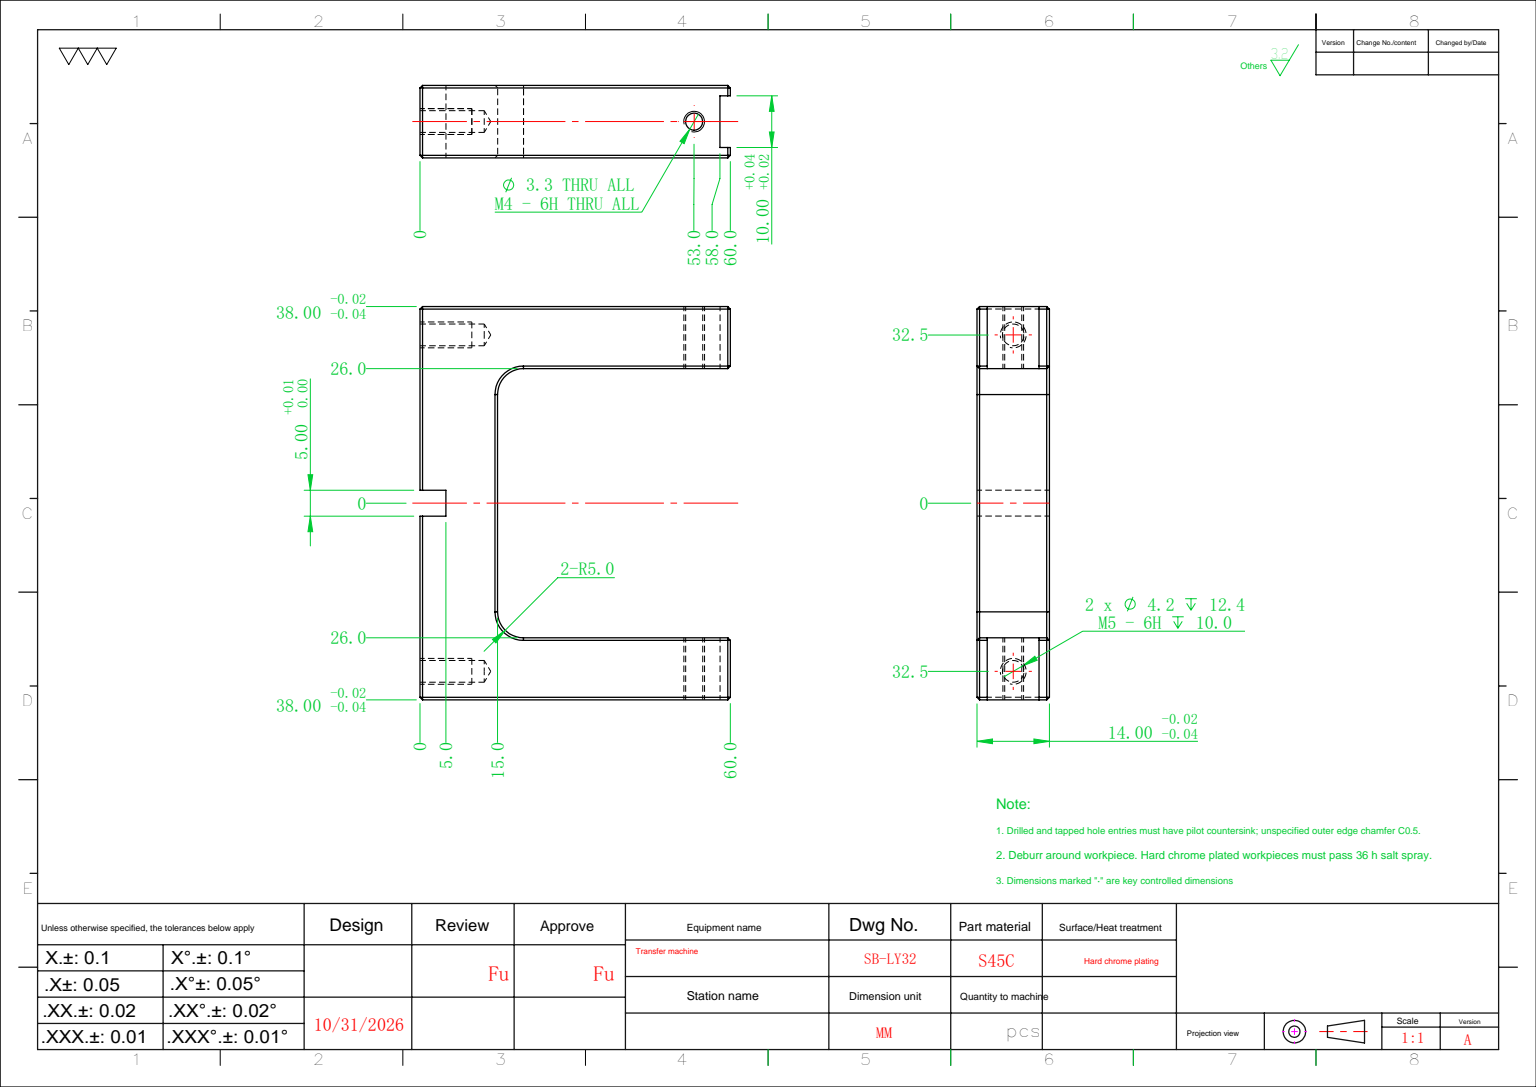
SolidWorks part; units mm, degrees
ref_plane "前视基准面" through (0, 0, 0) normal (0, 0, 1) x (1, 0, 0)
ref_plane "上视基准面" through (0, 0, 0) normal (0, 1, 0) x (1, 0, 0)
ref_plane "右视基准面" through (0, 0, 0) normal (1, 0, 0) x (0, 0, -1)
sketch "草图1" plane through (0, 0, 0) normal (0, 0, 1) x (1, 0, 0)
  line L1 (-30, -38) -> (30, -38)
  line L2 (-30, -38) -> (-30, 38)
  line L3 (-30, 38) -> (30, 38)
  line L4 (30, -38) -> (30, 38)
  line L5 (-30, -38) -> (30, 38) construction
  line L6 (-30, 38) -> (30, -38) construction
  point P0 (0, 0)
  dimension "D1" = 60
  dimension "D2" = 76
extrude "凸台-拉伸1" add sketch "草图1" along normal blind 14
sketch "草图2" plane through (0, 38, 0) normal (0, 1, 0) x (1, 0, 0)
  line L0 (30, -14) -> (30, 0) construction
  line L1 (30, -12) -> (28, -12)
  line L2 (30, -12) -> (30, -2)
  line L3 (30, -2) -> (28, -2)
  line L4 (28, -12) -> (28, -2)
  line L5 (30, -7) -> (19.2923, -7) construction
  dimension "D1" = 10
  dimension "D2" = 2
extrude "切除-拉伸1" cut sketch "草图2" against normal through all
sketch "草图3" plane through (0, 0, 0) normal (0, 0, -1) x (-1, 0, 0)
  line L0 (-30, -38) -> (-30, 38) construction
  line L1 (-30, -26) -> (15, -26)
  line L2 (-30, -26) -> (-30, 26)
  line L3 (-30, 26) -> (15, 26)
  line L4 (15, -26) -> (15, 26)
  line L5 (0, 0) -> (-71.3957, 0) construction
  line L6 (30, -38) -> (-30, -38) construction
  line L7 (30, 38) -> (30, -38) construction
  dimension "D1" = 12
  dimension "D2" = 15
extrude "切除-拉伸2" cut sketch "草图3" against normal through all
hole_wizard "M4 螺纹孔1" positions "草图4" profile "草图5" tap size "M4" standard "ISO" end condition through all
sketch "草图4" plane through (0, 38, 0) normal (0, 1, 0) x (1, 0, 0)
  line L0 (28, -7) -> (21.9058, -7) construction
  line L1 (28, -2) -> (28, -12) construction
  point P0 (23, -7)
  dimension "D1" = 5
sketch "草图5" plane through (23, 38, 7) normal (1, 0, 0) x (0, 0, 1)
  line L0 (0, 0) -> (0, 76)
  line L1 (0, 76) -> (1.65, 76)
  line L2 (1.65, 76) -> (1.65, 0)
  line L5 (1.65, 0) -> (0, 0)
  line L11 (0, -6.35) -> (0, 107.95) construction
  dimension "通孔螺纹孔钻头直径" = 3.3
  dimension "通孔螺纹孔钻头深度" = 76
cosmetic thread "孔螺蚊线1" parameters "D2"=4
hole_wizard "M5 螺纹孔2" positions "草图6" profile "草图7" tap size "M5" standard "ISO"
sketch "草图6" plane through (-30, 0, 0) normal (-1, 0, 0) x (0, 0, 1)
  line L0 (7, -38) -> (7, 38) construction
  line L1 (14, -38) -> (0, -38) construction
  line L2 (14, 38) -> (0, 38) construction
  line L4 (0, 0) -> (14, 0) construction
  line L5 (14, 38) -> (14, -38) construction
  point P0 (7, 32.5)
  point P3 (7, -32.5)
  dimension "D1" = 65
sketch "草图7" plane through (-30, 32.5, 7) normal (0, 1, 0) x (0, 0, 1)
  line L0 (0, 0) -> (0, 13.6618)
  line L1 (0, 13.6618) -> (2.1, 12.4)
  line L2 (2.1, 12.4) -> (2.1, 0)
  line L5 (2.1, 0) -> (0, 0)
  line L10 (0, 13.6618) -> (-2.1, 12.4) construction
  line L11 (0, -6.35) -> (0, 107.95) construction
  dimension "螺纹孔钻头直径" = 4.2
  dimension "螺纹孔钻头深度" = 12.4
  dimension "导头角度" = 118
cosmetic thread "孔螺蚊线2" parameters "D1"=10, "D2"=5
cosmetic thread "孔螺蚊线3" parameters "D1"=10, "D2"=5
sketch "草图8" plane through (0, 0, 14) normal (0, 0, 1) x (1, 0, 0)
  line L0 (-30, 38) -> (-30, -38) construction
  line L1 (-30, -2.5) -> (-25, -2.5)
  line L2 (-30, -2.5) -> (-30, 2.5)
  line L3 (-30, 2.5) -> (-25, 2.5)
  line L4 (-25, -2.5) -> (-25, 2.5)
  line L5 (-30, 0) -> (-16.3963, 0) construction
  dimension "D1" = 5
  dimension "D2" = 5
extrude "切除-拉伸3" cut sketch "草图8" against normal through all
fillet "圆角1" radius 5 2 edges at (-15, 26, 7) (-15, -26, 7)
chamfer "倒角1" distance 0.5 angle 45 32 edges at (10, 26, 0) (10, 26, 14) (-13.5355, 24.5355, 0) (-13.5355, 24.5355, 14) (-15, 0, 0) (-15, 0, 14) (-13.5355, -24.5355, 0) (-13.5355, -24.5355, 14) (-30, -20.25, 0) (30, -26, 1) (30, -38, 1) (10, -26, 0) (30, -32, 0) (0, -38, 0) (-30, -38, 7) (30, -26, 13) (30, -38, 13) (10, -26, 14) (30, -32, 14) (0, -38, 14) (-30, -20.25, 14) (30, 26, 1) (30, 38, 1) (30, 38, 13) (30, 26, 13) (-30, 20.25, 0) (30, 32, 0) (0, 38, 0) (-30, 38, 7) (30, 32, 14) (-30, 20.25, 14) (0, 38, 14)
